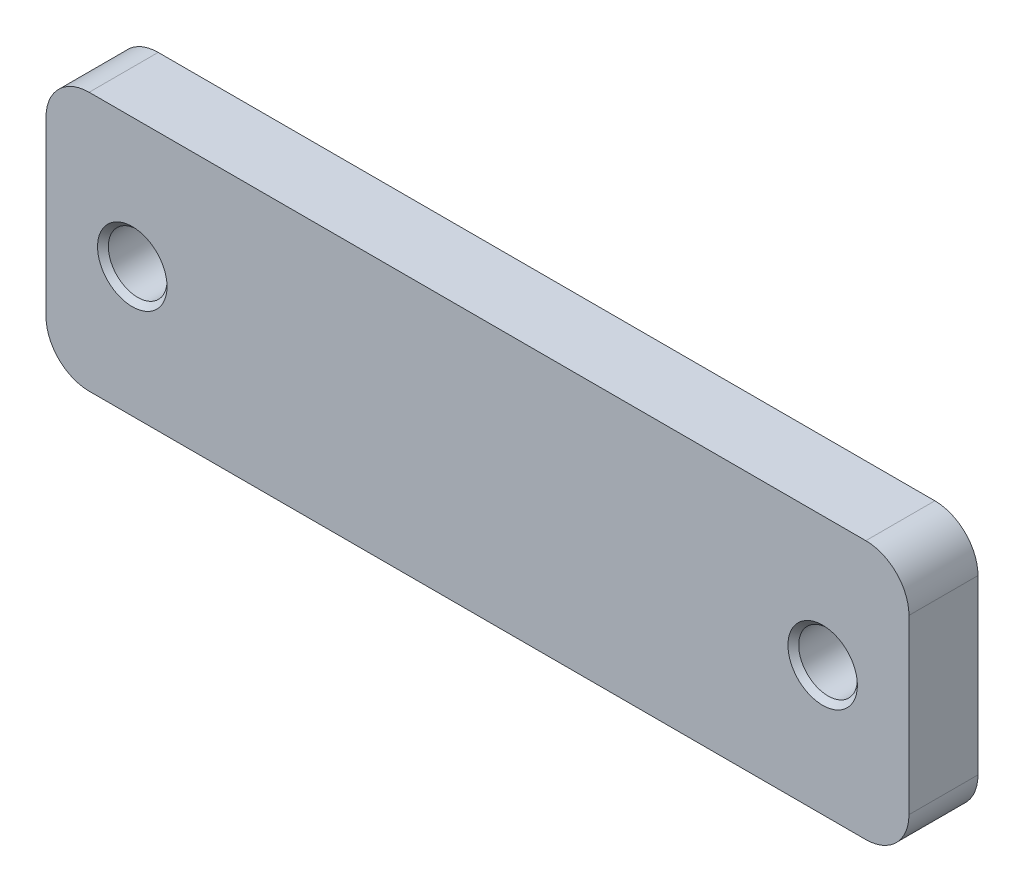
from build123d import *

# Parameters (mm, degrees)
SKETCH1_W                   = 100
SKETCH1_H                   = 30
BOSS_EXTRUDE1_DEPTH         = 8
FILLET1_R                   = 5
M8_TAPPED_HOLE1_D           = 6.8
M8_TAPPED_HOLE1_CSINK_D     = 8.05
M8_TAPPED_HOLE1_CSINK_ANGLE = 90


with BuildPart() as part:
    # Sketch1 → Boss-Extrude1 (new body)
    with BuildSketch(Plane.XY):
        Rectangle(SKETCH1_W, SKETCH1_H)
    extrude(amount=BOSS_EXTRUDE1_DEPTH)

    # Fillet1
    fillet1_edges = [part.edges().sort_by_distance(p)[0] for p in [
        (50, -15, 4),
        (-50, -15, 4),
        (-50, 15, 4),
        (50, 15, 4),
    ]]
    fillet(fillet1_edges, radius=FILLET1_R)

    # M8 Tapped Hole1 (through all)
    with Locations(Plane.XY.offset(8)):
        with Locations((-40, 0), (40, 0)):
            CounterSinkHole(M8_TAPPED_HOLE1_D / 2, M8_TAPPED_HOLE1_CSINK_D / 2, counter_sink_angle=M8_TAPPED_HOLE1_CSINK_ANGLE)


solid = part.part
